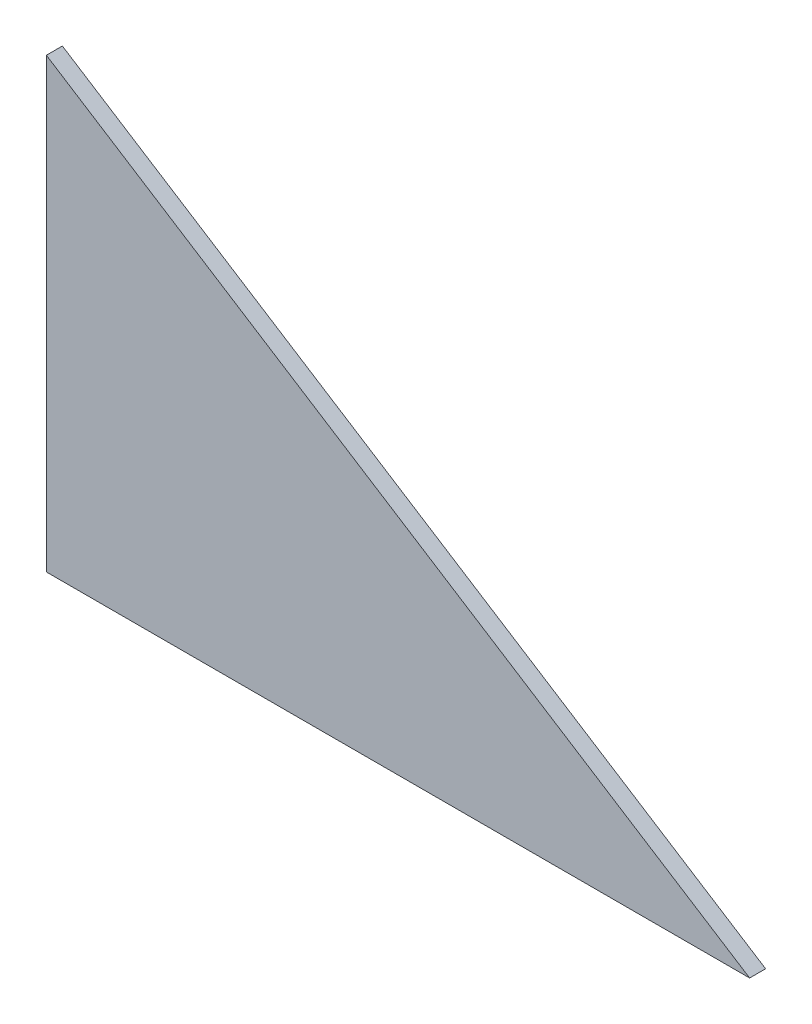
from build123d import *

# Parameters (mm, degrees)
BOSS_EXTRUDE1_DEPTH = 10


with BuildPart() as part:
    # Sketch1 → Boss-Extrude1 (new body)
    with BuildSketch(Plane.XY):
        Polygon((0, 0), (0, 280), (440, 0), align=None)
    extrude(amount=BOSS_EXTRUDE1_DEPTH)


solid = part.part
